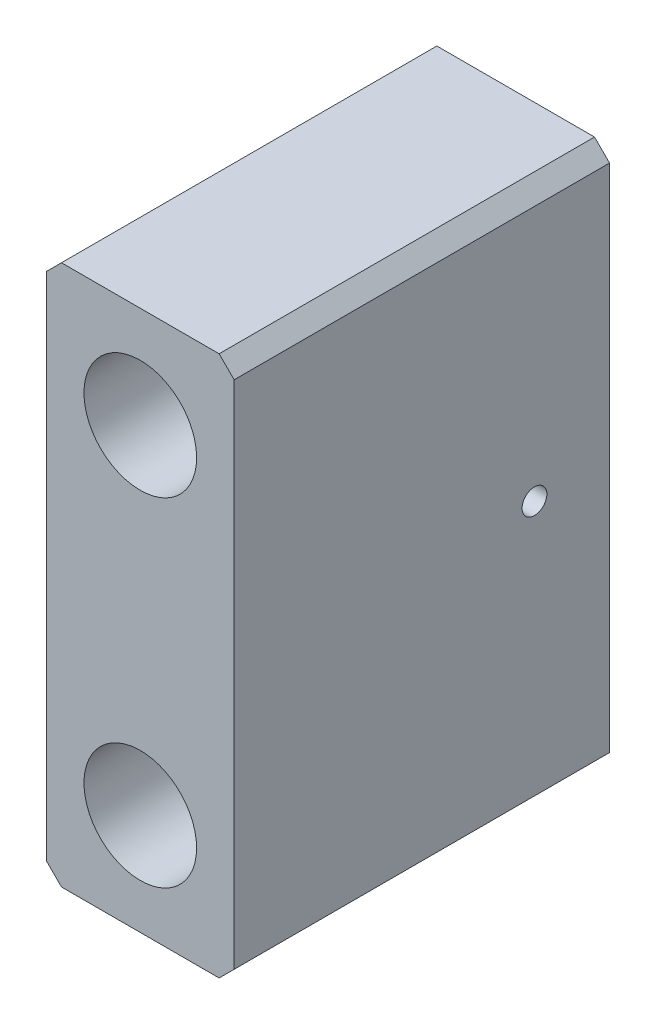
from build123d import *

# Parameters (mm, degrees)
SKETCH_1_W             = 25
SKETCH_1_H             = 72
SKETCH_1_R             = 7.5
EXTRUDE_1_DEPTH        = 50
HOLE_WIZARD_M4_1_D     = 3.3
HOLE_WIZARD_M4_1_DEPTH = 8.1
HOLE_WIZARD_M4_1_TIP   = 0.991420021
CHAMFER_1_SIZE         = 2


with BuildPart() as part:
    # 草图1 → 凸台-拉伸1 (new body)
    with BuildSketch(Plane.XY):
        Rectangle(SKETCH_1_W, SKETCH_1_H)
        with Locations((0, 22.5)):
            Circle(SKETCH_1_R, mode=Mode.SUBTRACT)
        with Locations((0, -22.5)):
            Circle(SKETCH_1_R, mode=Mode.SUBTRACT)
    extrude(amount=EXTRUDE_1_DEPTH)

    # M4 螺纹孔1
    with Locations(Plane(origin=(12.5, 0, 10), x_dir=(0, 0, 1), z_dir=(1, 0, 0))):
        with Locations((0, 0)):
            Hole(HOLE_WIZARD_M4_1_D / 2, depth=HOLE_WIZARD_M4_1_DEPTH)
            with Locations((0, 0, -(HOLE_WIZARD_M4_1_DEPTH + HOLE_WIZARD_M4_1_TIP / 2))):  # 118° drill point
                Cone(0, HOLE_WIZARD_M4_1_D / 2, HOLE_WIZARD_M4_1_TIP, mode=Mode.SUBTRACT)

    # 倒角1
    chamfer_1_edges = [part.edges().sort_by_distance(p)[0] for p in [
        (12.5, -36, 25),
        (-12.5, -36, 25),
        (-12.5, 36, 25),
        (12.5, 36, 25),
    ]]
    chamfer(chamfer_1_edges, length=CHAMFER_1_SIZE)


solid = part.part
